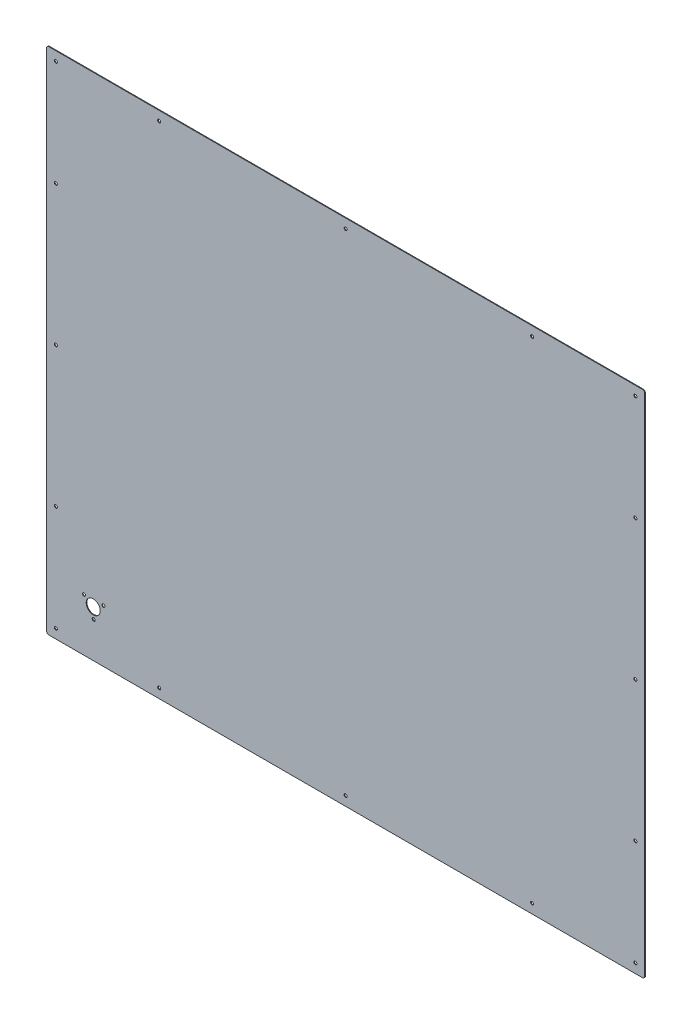
SolidWorks part; units mm, degrees
material "不锈钢 (铁素体)"
ref_plane "主视基准图" through (0, 0, 0) normal (0, 0, 1) x (1, 0, 0)
ref_plane "上视基准图" through (0, 0, 0) normal (0, 1, 0) x (1, 0, 0)
ref_plane "右视基准图" through (0, 0, 0) normal (1, 0, 0) x (0, 0, -1)
sketch "草图1" plane through (0, 0, 0) normal (0, 0, 1) x (1, 0, 0)
  line L0 (-641.5, 546.5) -> (641.5, 546.5)
  line L1 (-642.5, -547.5) -> (642.5, -547.5) construction
  line L2 (-642.5, -547.5) -> (-642.5, 547.5) construction
  line L3 (-642.5, 547.5) -> (642.5, 547.5) construction
  line L4 (642.5, -547.5) -> (642.5, 547.5) construction
  line L5 (-642.5, -547.5) -> (642.5, 547.5) construction
  line L6 (-642.5, 547.5) -> (642.5, -547.5) construction
  line L7 (641.5, -546.5) -> (641.5, 546.5)
  line L8 (-641.5, -546.5) -> (641.5, -546.5)
  line L9 (-641.5, -546.5) -> (-641.5, 546.5)
  point P0 (0, 0)
  dimension "D1" = 1285
  dimension "D2" = 1095
  dimension "D3" = 1
extrude "凸台-拉伸1" add sketch "草图1" along normal blind 1.5
fillet "圆角1" radius 5 4 edges at (641.5, 546.5, 0.75) (641.5, -546.5, 0.75) (-641.5, -546.5, 0.75) (-641.5, 546.5, 0.75)
hole_wizard "Ø6.5 (6.5) 直径孔1" positions "草图4" profile "草图3" hole size "Ø6.5" standard "Ansi Metric"
sketch "草图4" plane through (0, 0, 1.5) normal (0, 0, 1) x (1, 0, 0)
  line L0 (0, 0) -> (0, -207.5721) construction
  line L1 (0, 0) -> (177.7731, 0) construction
  point P0 (0, 526.5)
  point P2 (400, 526.5)
  point P4 (-400, 526.5)
  point P6 (-621.5, 300)
  point P8 (-621.5, 0)
  point P10 (-621.5, -300)
  point P12 (-400, -526.5)
  point P14 (0, -526.5)
  point P16 (400, -526.5)
  point P18 (621.5, 300)
  point P20 (621.5, 0)
  point P22 (621.5, -300)
  point P33 (-621.5, 526.5)
  point P35 (-621.5, -526.5)
  point P37 (621.5, -526.5)
  point P39 (621.5, 526.5)
  dimension "D1" = 1243
  dimension "D2" = 1053
  dimension "D3" = 800
  dimension "D4" = 600
sketch "草图3" plane through (0, 526.5, 1.5) normal (1, 0, 0) x (0, -1, 0)
  line L0 (0, 0) -> (0, 17.4864)
  line L1 (0, 17.4864) -> (3.25, 15.61)
  line L2 (3.25, 15.61) -> (3.25, 0)
  line L5 (3.25, 0) -> (0, 0)
  line L10 (0, 17.4864) -> (-3.25, 15.61) construction
  line L11 (0, -6.35) -> (0, 107.95) construction
  dimension "孔直径" = 6.5
  dimension "孔深度" = 15.61
  dimension "导头角度" = 120
sketch "草图5" plane through (0, 0, 1.5) normal (0, 0, 1) x (1, 0, 0)
  line L0 (-636.5, -546.5) -> (636.5, -546.5) construction
  line L1 (-641.5, 541.5) -> (-641.5, -541.5) construction
  circle A0 centre (-541.5, -446.5) radius 15
  dimension "D1" = 30
  dimension "D2" = 100
  dimension "D3" = 100
extrude "切除-拉伸1" cut sketch "草图5" against normal blind 10
hole_wizard "Ø6.5 (6.5) 直径孔2" positions "草图7" profile "草图6" hole size "Ø6.5" standard "Ansi Metric"
sketch "草图7" plane through (0, 0, 1.5) normal (0, 0, 1) x (1, 0, 0)
  point P0 (-561.2846, -433.5)
  point P3 (-540.5, -469.5)
  point P6 (-519.7154, -433.5)
sketch "草图6" plane through (-561.2846, -433.5, 1.5) normal (1, 0, 0) x (0, -1, 0)
  line L0 (0, 0) -> (0, 17.4864)
  line L1 (0, 17.4864) -> (3.25, 15.61)
  line L2 (3.25, 15.61) -> (3.25, 0)
  line L5 (3.25, 0) -> (0, 0)
  line L10 (0, 17.4864) -> (-3.25, 15.61) construction
  line L11 (0, -6.35) -> (0, 107.95) construction
  dimension "孔直径" = 6.5
  dimension "孔深度" = 15.61
  dimension "导头角度" = 120
